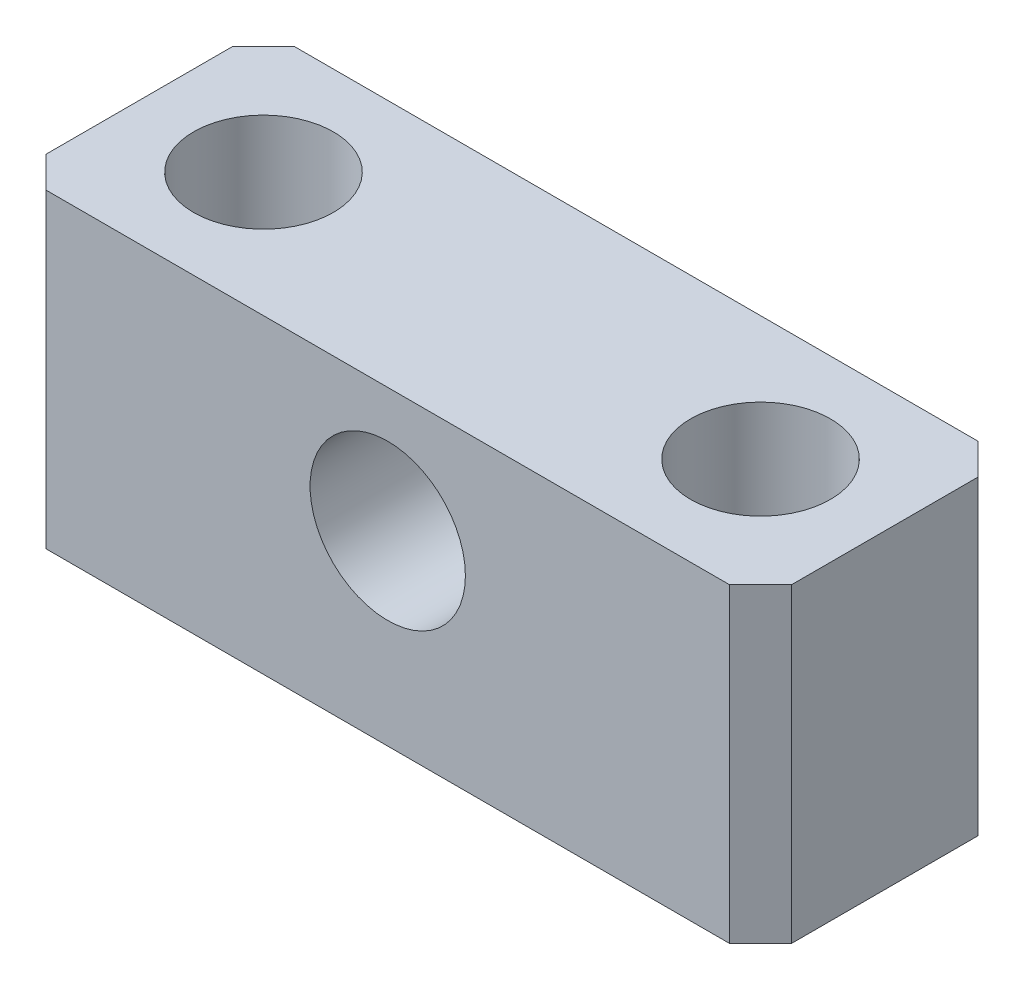
SolidWorks part; units mm, degrees
ref_plane "Front Plane" through (0, 0, 0) normal (0, 0, 1) x (1, 0, 0)
ref_plane "Top Plane" through (0, 0, 0) normal (0, 1, 0) x (1, 0, 0)
ref_plane "Right Plane" through (0, 0, 0) normal (1, 0, 0) x (0, 0, -1)
sketch "Sketch1" plane through (0, 0, 0) normal (0, 0, 1) x (1, 0, 0)
  line L1 (-12, 5) -> (12, 5)
  line L2 (-12, 5) -> (-12, -5)
  line L3 (-12, -5) -> (12, -5)
  line L4 (12, 5) -> (12, -5)
  line L5 (-12, 5) -> (12, -5) construction
  line L6 (-12, -5) -> (12, 5) construction
  point P0 (0, 0)
  dimension "D1" = 10
  dimension "D2" = 24
extrude "Boss-Extrude1" add sketch "Sketch1" along normal mid plane 8
hole_wizard "Ø4.5 (4.5) Diameter Hole1" positions "Sketch3" profile "Sketch2" hole size "Ø4.5" standard "Gb" end condition through all
sketch "Sketch3" plane through (0, 5, 0) normal (0, 1, 0) x (1, 0, 0)
  line L0 (0, 0) -> (0, 5.3207) construction
  point P0 (-8, 0)
  point P2 (8, 0)
  dimension "D1" = 16
sketch "Sketch2" plane through (-8, 5, 0) normal (1, 0, 0) x (0, 0, 1)
  line L0 (0, 0) -> (0, 10)
  line L1 (0, 10) -> (2.25, 10)
  line L2 (2.25, 10) -> (2.25, 0)
  line L5 (2.25, 0) -> (0, 0)
  line L11 (0, -6.35) -> (0, 107.95) construction
  dimension "通孔孔直径" = 4.5
  dimension "通孔孔深度" = 10
chamfer "Chamfer1" distance 1 angle 45 4 edges at (-12, 0, -4) (12, 0, -4) (12, 0, 4) (-12, 0, 4)
hole_wizard "Ø5.0 (5) Diameter Hole1" positions "Sketch6" profile "Sketch5" hole size "Ø5.0" standard "Gb" end condition through all
sketch "Sketch6" plane through (0, 0, 4) normal (0, 0, 1) x (1, 0, 0)
  line L0 (11, 5) -> (-11, 5) construction
  point P0 (0, 1)
  dimension "D1" = 4
sketch "Sketch5" plane through (0, 1, 4) normal (1, 0, 0) x (0, -1, 0)
  line L0 (0, 0) -> (0, 8)
  line L1 (0, 8) -> (2.5, 8)
  line L2 (2.5, 8) -> (2.5, 0)
  line L5 (2.5, 0) -> (0, 0)
  line L11 (0, -6.35) -> (0, 107.95) construction
  dimension "通孔孔直径" = 5
  dimension "通孔孔深度" = 8
